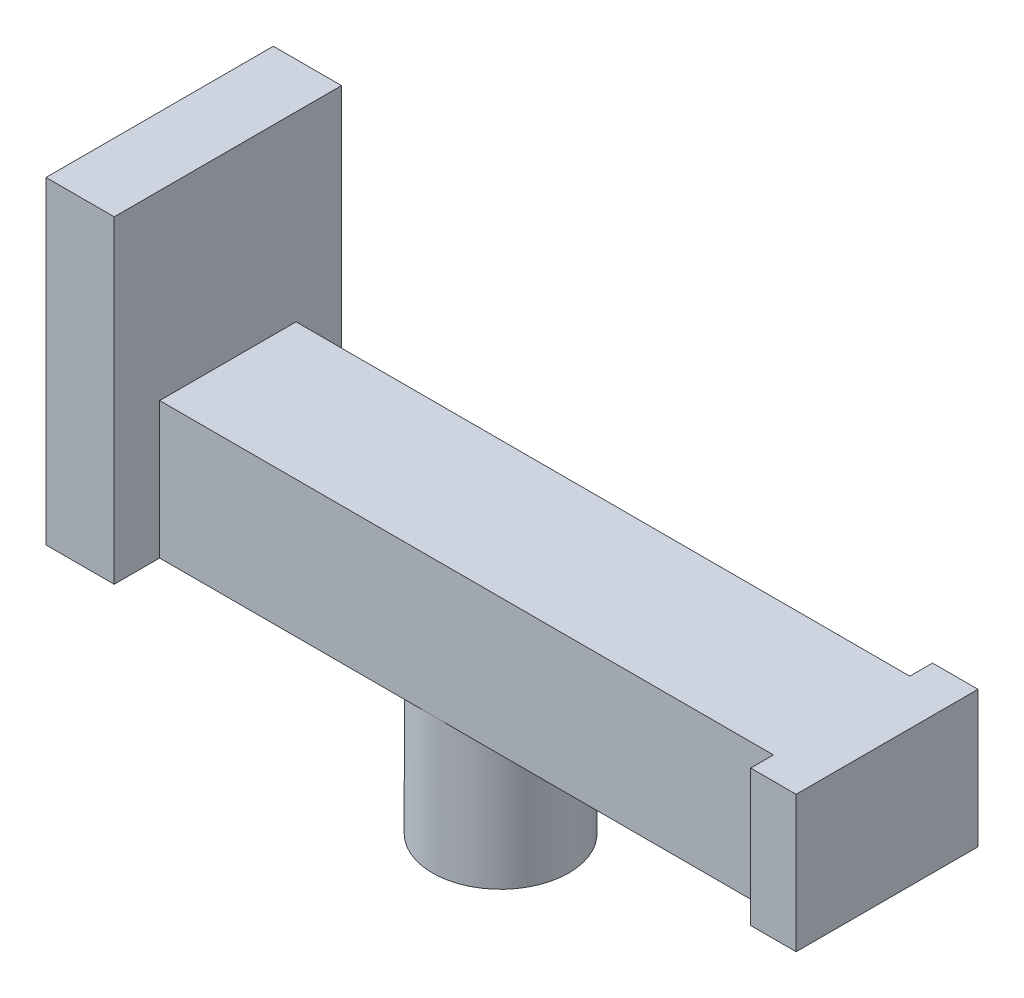
from build123d import *

# Parameters (mm, degrees)
SKETCH1_W           = 50
SKETCH1_H           = 6
BOSS_EXTRUDE1_DEPTH = 6
SKETCH2_R           = 3
BOSS_EXTRUDE2_DEPTH = 6
SKETCH3_W           = 10
SKETCH3_H           = 6
BOSS_EXTRUDE3_DEPTH = 3
SKETCH4_W           = 6
SKETCH4_H           = 6
CUT_EXTRUDE1_DEPTH  = 20
SKETCH5_W           = 8
SKETCH5_H           = 6
BOSS_EXTRUDE4_DEPTH = 2
SKETCH6_W           = 3
SKETCH6_H           = 10
BOSS_EXTRUDE5_DEPTH = 8


with BuildPart() as part:
    # Sketch1 → Boss-Extrude1 (new body)
    with BuildSketch(Plane.XY):
        Rectangle(SKETCH1_W, SKETCH1_H)
    extrude(amount=BOSS_EXTRUDE1_DEPTH)

    # Sketch2 → Boss-Extrude2 (add)
    with BuildSketch(Plane.XZ.offset(3)):
        with Locations(Location((-10, 3, 0), (0, 0, 270))):
            Circle(SKETCH2_R)
    extrude(amount=BOSS_EXTRUDE2_DEPTH)

    # Sketch3 → Boss-Extrude3 (add)
    with BuildSketch(Plane.ZY.offset(25)):
        with Locations((3, 0)):
            Rectangle(SKETCH3_W, SKETCH3_H)
    extrude(amount=-BOSS_EXTRUDE3_DEPTH)

    # Sketch4 → Cut-Extrude1 (cut)
    with BuildSketch(Plane(origin=(25, 0, 0), x_dir=(0, 0, -1), z_dir=(1, 0, 0))):
        with Locations((-3, 0)):
            Rectangle(SKETCH4_W, SKETCH4_H)
    extrude(amount=-CUT_EXTRUDE1_DEPTH, mode=Mode.SUBTRACT)

    # Sketch5 → Boss-Extrude4 (add)
    with BuildSketch(Plane(origin=(5, 0, 0), x_dir=(0, 0, -1), z_dir=(1, 0, 0))):
        with Locations((-3, 0)):
            Rectangle(SKETCH5_W, SKETCH5_H)
    extrude(amount=BOSS_EXTRUDE4_DEPTH)

    # Sketch6 → Boss-Extrude5 (add)
    with BuildSketch(Plane(origin=(0, 3, 0), x_dir=(1, 0, 0), z_dir=(0, 1, 0))):
        with Locations((-23.5, -3)):
            Rectangle(SKETCH6_W, SKETCH6_H)
    extrude(amount=BOSS_EXTRUDE5_DEPTH)


solid = part.part
